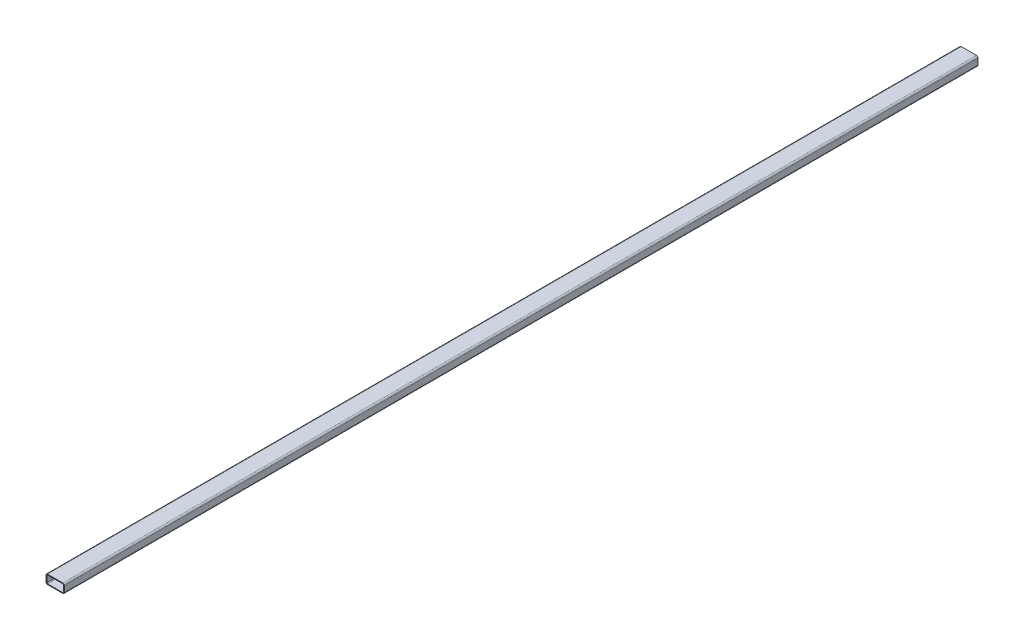
SolidWorks part; units mm, degrees
material "普通碳钢"
ref_plane "Front Plane" through (0, 0, 0) normal (0, 0, 1) x (1, 0, 0)
ref_plane "Top Plane" through (0, 0, 0) normal (0, 1, 0) x (1, 0, 0)
ref_plane "Right Plane" through (0, 0, 0) normal (1, 0, 0) x (0, 0, -1)
sketch "Sketch1" plane through (0, 0, 0) normal (0, 0, 1) x (1, 0, 0)
  line L0 (10, 55) -> (110, 55)
  line L1 (10, 0) -> (110, 0)
  line L2 (0, 10) -> (0, 50)
  line L3 (10, 60) -> (110, 60)
  line L4 (120, 10) -> (120, 50)
  line L5 (115, 10) -> (115, 50)
  line L6 (10, 5) -> (110, 5)
  line L7 (5, 10) -> (5, 50)
  arc A0 (120, 10) -> (110, 0) centre (110, 10) cw
  arc A1 (0, 50) -> (10, 60) centre (10, 50) cw
  arc A2 (120, 50) -> (110, 60) centre (110, 50) ccw
  arc A3 (10, 0) -> (0, 10) centre (10, 10) cw
  arc A4 (115, 50) -> (110, 55) centre (110, 50) ccw
  arc A5 (115, 10) -> (110, 5) centre (110, 10) cw
  arc A6 (10, 5) -> (5, 10) centre (10, 10) cw
  arc A7 (5, 50) -> (10, 55) centre (10, 50) cw
  point P7 (120, 0)
  point P10 (0, 60)
  point P13 (120, 60)
  point P16 (0, 0)
  dimension "D3" = 10
  dimension "D4" = 10
  dimension "D5" = 10
  dimension "D6" = 10
  dimension "D1" = 120
  dimension "D2" = 60
  dimension "D7" = 5
extrude "Boss-Extrude1" add sketch "Sketch1" along normal blind 6000
